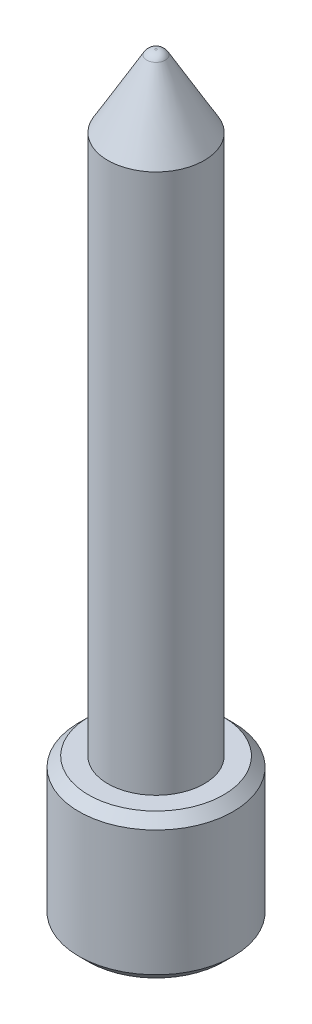
from build123d import *

# Parameters (mm, degrees)
CHAMFER1_SIZE = 1


with BuildPart() as part:
    # Sketch1 → Revolve1 (revolve)
    with BuildSketch(Plane.XY, mode=Mode.PRIVATE) as revolve1_sk:
        with BuildLine():
            Line((-0.96339526, 77.991604501), (-5, 71))
            Line((-5, 71), (-5, 15))
            Line((-5, 15), (-8, 15))
            Line((-8, 15), (-8, 0))
            Line((-8, 0), (0, 0))
            Line((0, 0), (0, 78.491604501))
            Line((0, 78.491604501), (-0.097369856, 78.491604501))
            ThreePointArc((-0.097369856, 78.491604501), (-0.597369856, 78.357629904), (-0.96339526, 77.991604501))
        make_face()
    revolve(revolve1_sk.sketch.rotate(Axis((0, 0, 0), (0, 1, 0)), 270), axis=Axis((0, 0, 0), (0, 1, 0)))

    # Chamfer1
    chamfer1_edges = [part.edges().sort_by_distance(p)[0] for p in [
        (0, 0, 8),
        (0, 15, 8),
    ]]
    chamfer(chamfer1_edges, length=CHAMFER1_SIZE)


solid = part.part
